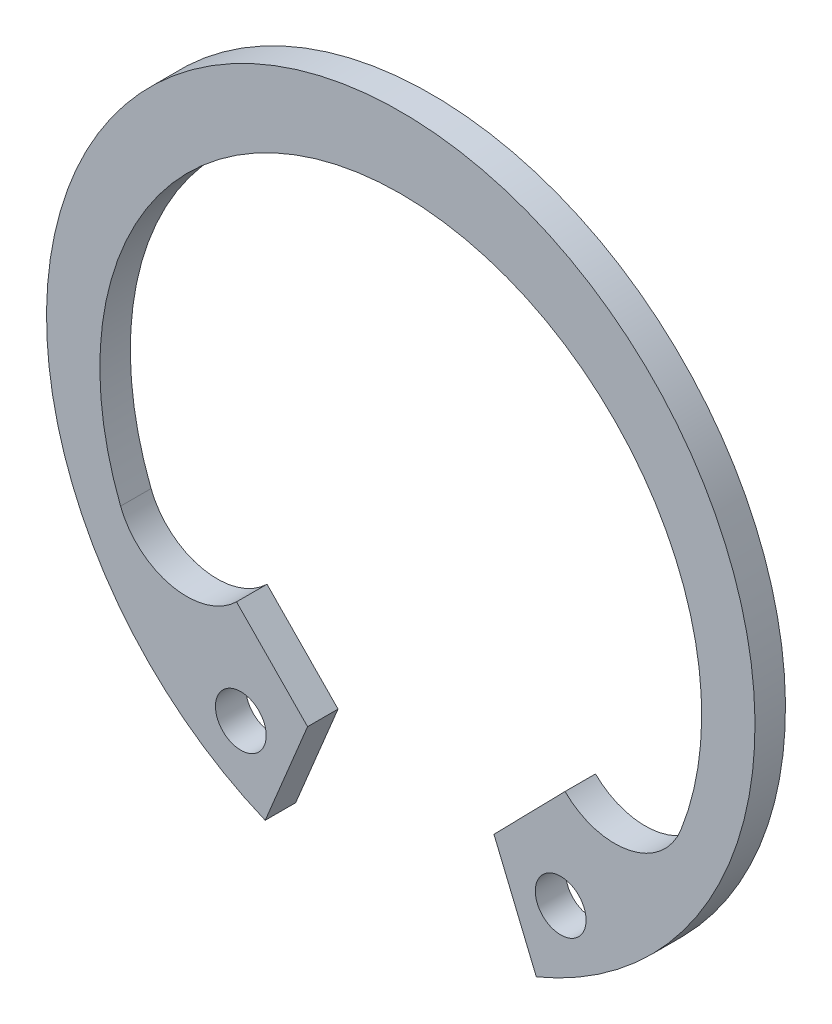
from build123d import *

# Parameters (mm, degrees)
SKETCH_1_R        = 1
EXTRUDE_952_DEPTH = 1.2


with BuildPart() as part:
    # 草图1 → Extrude 952 (new body)
    with BuildSketch(Plane.XY):
        with BuildLine():
            Line((-6.468002299, -6.001541065), (-3.669934116, -8.860004717))
            Line((-3.669934116, -8.860004717), (-5.338433881, -12.888119479))
            ThreePointArc((-5.338433881, -12.888119479), (0, 13.95), (5.338433881, -12.888119479))
            Line((5.338433881, -12.888119479), (3.669934116, -8.860004717))
            Line((3.669934116, -8.860004717), (6.468002299, -6.001541065))
            ThreePointArc((6.468002299, -6.001541065), (9.014108926, -6.738296556), (11.033790366, -5.021801727))
            ThreePointArc((11.033790366, -5.021801727), (0, 11.15), (-11.033790366, -5.021801727))
            ThreePointArc((-11.033790366, -5.021801727), (-9.014108926, -6.738296556), (-6.468002299, -6.001541065))
        make_face()
        with Locations((-6.298089329, -9.978680815)):
            Circle(SKETCH_1_R, mode=Mode.SUBTRACT)
        with Locations(Location((6.298089329, -9.978680815, 0), (0, 0, 180))):
            Circle(SKETCH_1_R, mode=Mode.SUBTRACT)
    extrude(amount=EXTRUDE_952_DEPTH)


solid = part.part
